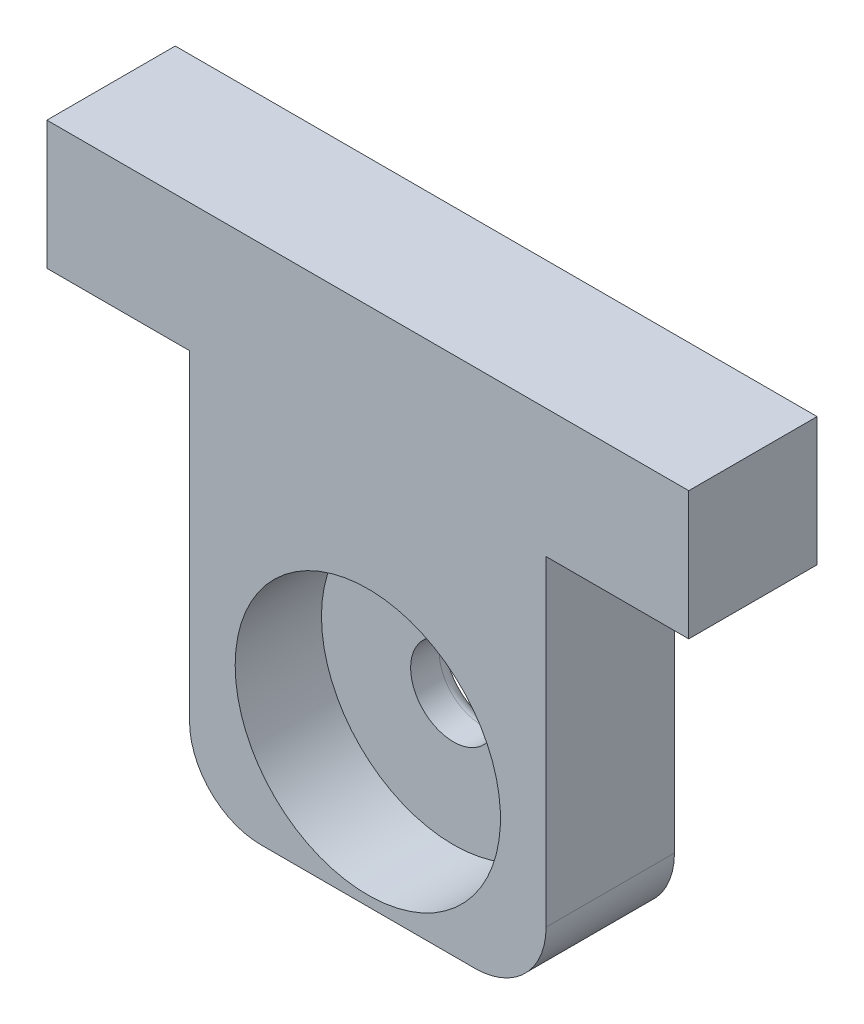
SolidWorks part; units mm, degrees
ref_plane "前视基准面" through (0, 0, 0) normal (0, 0, 1) x (1, 0, 0)
ref_plane "上视基准面" through (0, 0, 0) normal (0, 1, 0) x (1, 0, 0)
ref_plane "右视基准面" through (0, 0, 0) normal (1, 0, 0) x (0, 0, -1)
sketch "草图1" plane through (0, 0, 0) normal (0, 0, 1) x (1, 0, 0)
  line L1 (25, 60) -> (-25, 60)
  line L2 (25, 60) -> (25, -60)
  line L3 (25, -60) -> (-25, -60)
  line L4 (-25, 60) -> (-25, -60)
  line L5 (25, 60) -> (-25, -60) construction
  line L6 (25, -60) -> (-25, 60) construction
  point P0 (0, 0)
  dimension "D1" = 120
  dimension "D2" = 50
extrude "凸台-拉伸1" add sketch "草图1" along normal blind 18
sketch "草图2" plane through (0, 60, 0) normal (0, 1, 0) x (1, 0, 0)
  line L0 (25, 0) -> (-25, 0) construction
  line L1 (45, -18) -> (-45, -18)
  line L2 (45, -18) -> (45, 0)
  line L3 (45, 0) -> (-45, 0)
  line L4 (-45, -18) -> (-45, 0)
  line L5 (45, -18) -> (-45, 0) construction
  line L6 (45, 0) -> (-45, -18) construction
  line L7 (25, -18) -> (-25, -18) construction
  line L8 (0, -9) -> (0, 0) construction
  line L9 (-25, -18) -> (-25, 0) construction
  point P0 (0, -9)
  dimension "D1" = 20
extrude "凸台-拉伸2" add sketch "草图2" against normal blind 18
fillet "圆角1" radius 10 2 edges at (25, -60, 9) (-25, -60, 9)
sketch "草图3" plane through (0, 0, 0) normal (0, 0, -1) x (-1, 0, 0)
  line L0 (15, -60) -> (-15, -60) construction
  line L1 (0, 0) -> (0, -40) construction
  circle A0 centre (0, -40) radius 6
  dimension "D1" = 12
  dimension "D2" = 20
extrude "切除-拉伸1" cut sketch "草图3" against normal through all
sketch "草图4" plane through (0, 0, 0) normal (0, 0, -1) x (-1, 0, 0)
  circle A0 centre (0, -40) radius 18.5
  circle A1 centre (0, -40) radius 18.6
  dimension "D2" = 37
  dimension "D1" = 0.1
extrude "切除-拉伸2" cut sketch "草图4" against normal through all
pattern_linear "阵列(线性)1" count 2 spacing 47 along (0, 1, 0) of "切除-拉伸1", "切除-拉伸2"
fillet "圆角2" radius 2 4 edges at (-18.5, -40, 18) (-6, -40, 18) (-18.5, -40, 0) (-6, -40, 0)
fillet "圆角3" radius 2 4 edges at (-18.5, 7, 0) (-6, 7, 0) (-18.5, 7, 18) (-6, 7, 18)
sketch "草图5" plane through (0, 0, 0) normal (0, 0, -1) x (-1, 0, 0)
  line L0 (25, 42) -> (25, -50) construction
  line L1 (25, -13) -> (-30.7081, -13)
  line L2 (25, -13) -> (25, -61.0068)
  line L3 (25, -61.0068) -> (-30.7081, -61.0068)
  line L4 (-30.7081, -13) -> (-30.7081, -61.0068)
  line L5 (-45, 42) -> (-25, 42) construction
  dimension "D1" = 55
extrude "切除-拉伸3" cut sketch "草图5" against normal through all
fillet "圆角4" radius 10 2 edges at (25, -13, 9) (-25, -13, 9)
sketch "草图6" plane through (0, 0, 18) normal (0, 0, 1) x (1, 0, 0)
  circle A0 centre (0, 7) radius 18.6
extrude "切除-拉伸4" cut sketch "草图6" against normal blind 12
